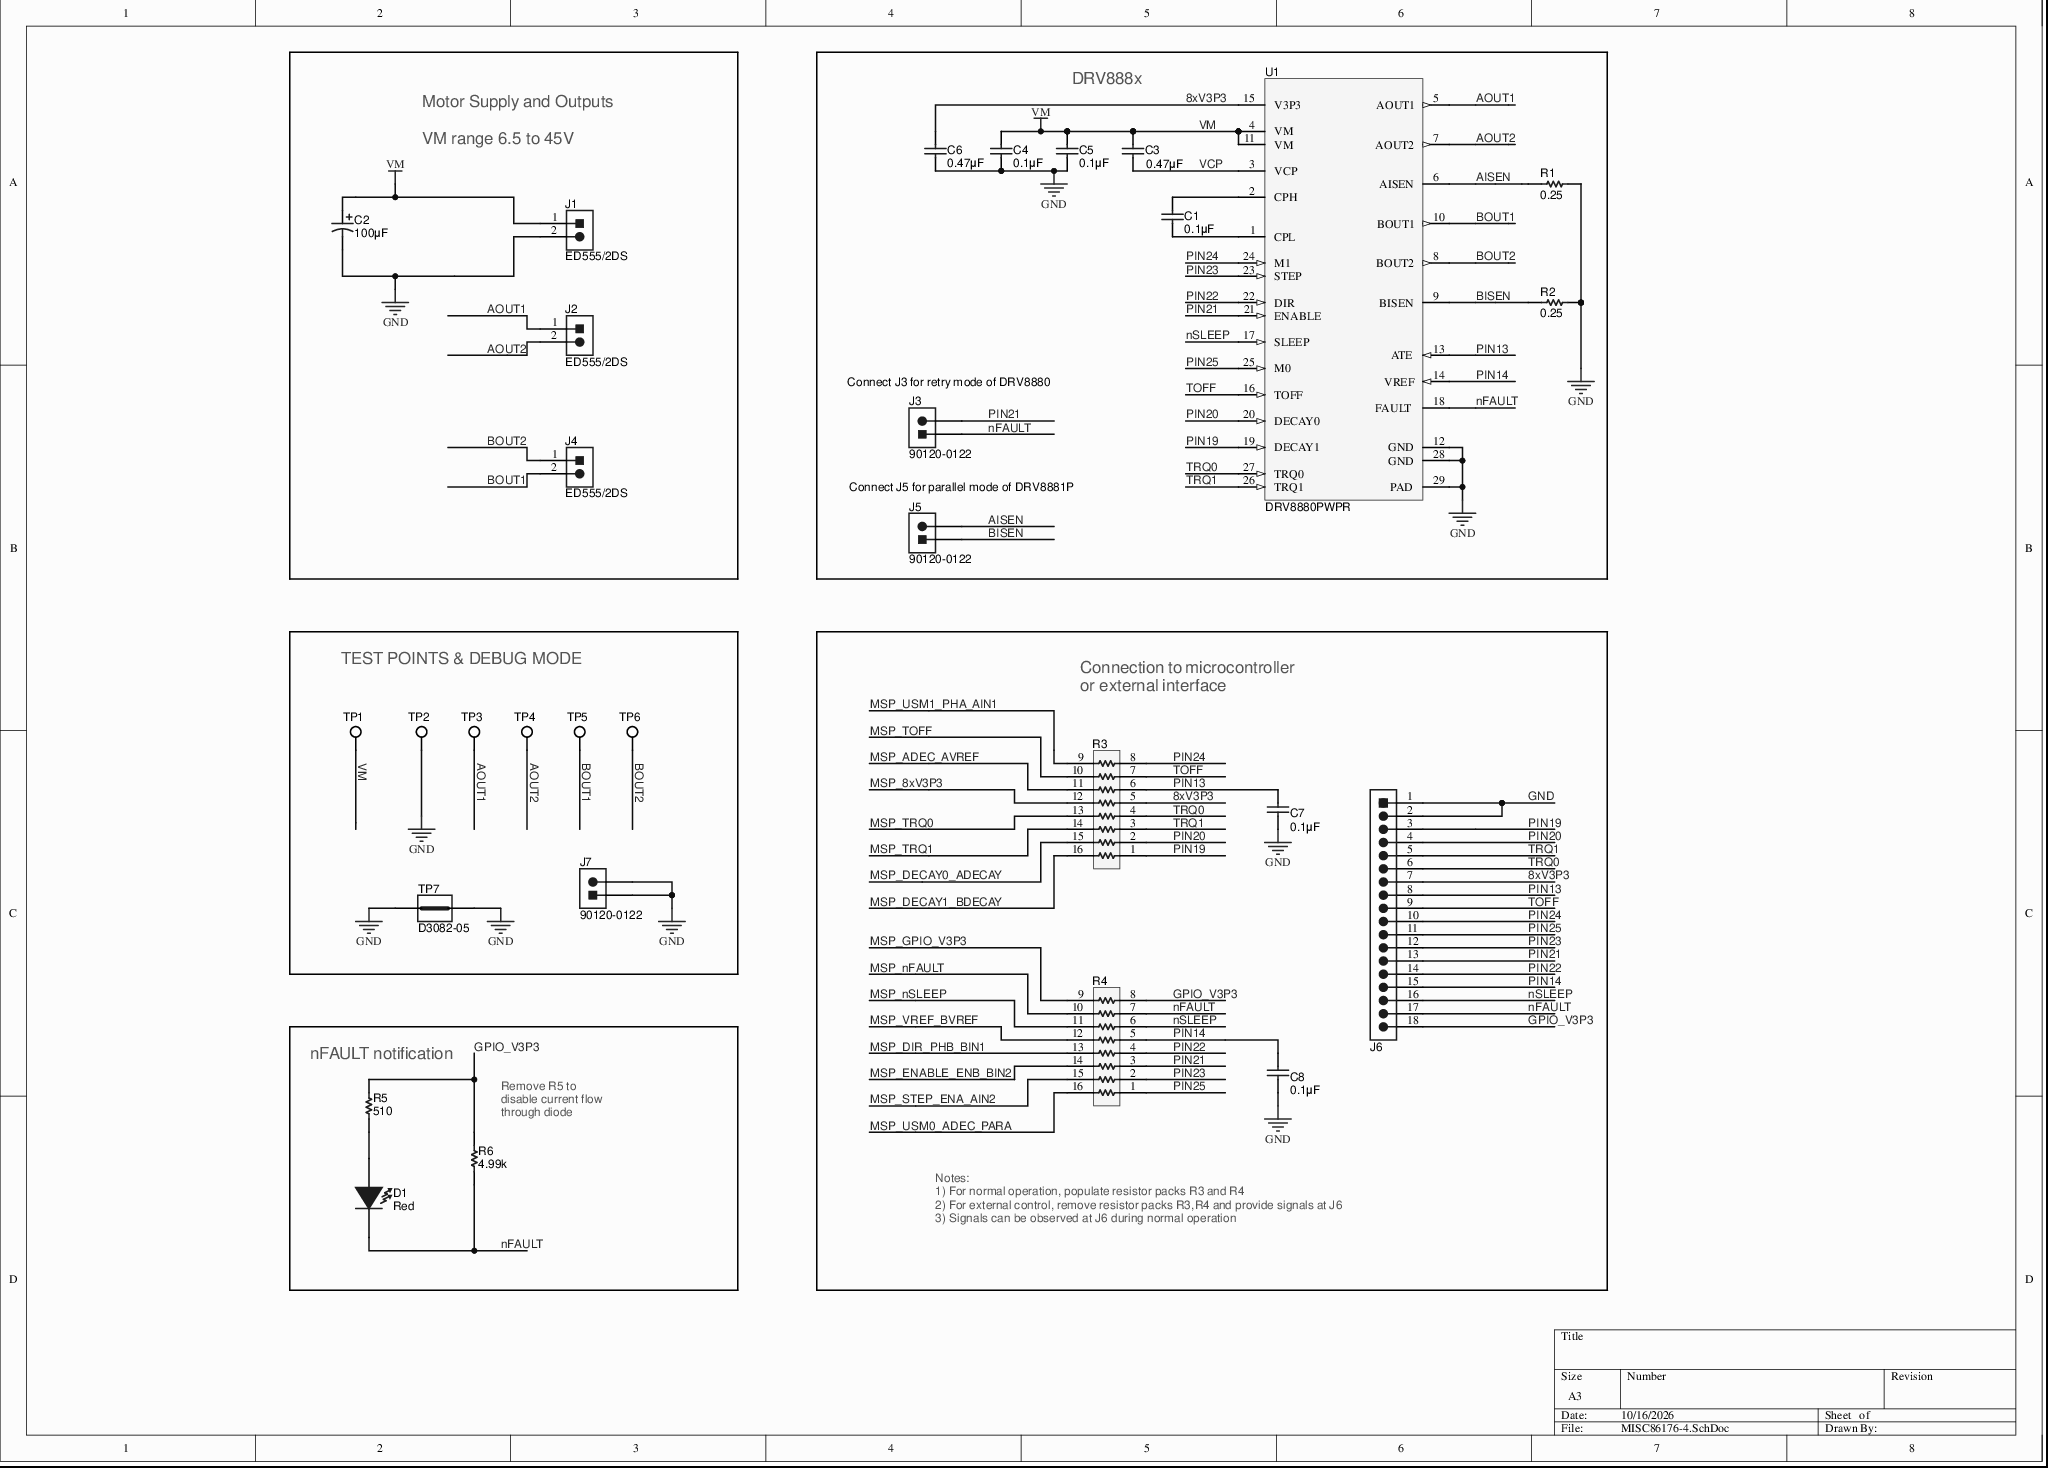
[diagram p0: MISC86176-4.SchDoc]
# Altium project MISC86176-2.PrjPCB
2 sheets, 47 parts. Net scope: global (net labels, ports and power ports of the same name join across sheets).
Board file: MISC86176.PcbDoc
Sheets:
  MISC86176-4.SchDoc
  MISC86176-6.SchDoc

## Sheet MISC86176-4.SchDoc
size A3

### Parts
C1  ValueDisplayed: 0.1µF  [0805L]  (hidden comment: C0805C104K1RACTU)
C2  ValueDisplayed: 100µF  [SM_RADIAL_G]  (hidden comment: EEE-FK1J101P)
C3  ValueDisplayed: 0.47µF  [0805L]  (hidden comment: C2012X7R1E474K)
C4  ValueDisplayed: 0.1µF  [0805L]  (hidden comment: C0805C104K1RACTU)
C5  ValueDisplayed: 0.1µF  [0805L]  (hidden comment: C0805C104K1RACTU)
C6  ValueDisplayed: 0.47µF  [0603L]  (hidden comment: C0603C474K9RACTU)
C7  ValueDisplayed: 0.1µF  [0402L]  (hidden comment: GRM155R61A104KA01D)
C8  ValueDisplayed: 0.1µF  [0402L]  (hidden comment: GRM155R61A104KA01D)
D1  value Red  [LED_LTST-C190_Red]  (hidden comment: LTST-C190CKT)
J1  ED555/2DS  [TERM_BLK_ED555-2DS]
J2  ED555/2DS  [TERM_BLK_ED555-2DS]
J3  90120-0122  [CONN_90120-0122]
J4  ED555/2DS  [TERM_BLK_ED555-2DS]
J5  90120-0122  [CONN_90120-0122]
J6  TSW-118-07-G-S  [TSW-118-07-G-S]  (value not drawn)
J7  90120-0122  [CONN_90120-0122]
R1  value 0.25  [2010L]  (hidden comment: CSRN2010FKR250)
R2  value 0.25  [2010L]  (hidden comment: CSRN2010FKR250)
R3  EXB-2HV330JV  [RESCAXS_EXB-2HV]  (value not drawn)
R4  EXB-2HV330JV  [RESCAXS_EXB-2HV]  (value not drawn)
R5  value 510  [0402L]  (hidden comment: CRCW0402510RJNED)
R6  value 4.99k  [0402L]  (hidden comment: CRCW04024K99FKED)
TP1  5016  [Testpoint_Keystone_Compact]  (value not drawn)
TP2  5016  [Testpoint_Keystone_Compact]  (value not drawn)
TP3  5016  [Testpoint_Keystone_Compact]  (value not drawn)
TP4  5016  [Testpoint_Keystone_Compact]  (value not drawn)
TP5  5016  [Testpoint_Keystone_Compact]  (value not drawn)
TP6  5016  [Testpoint_Keystone_Compact]  (value not drawn)
TP7  D3082-05  [Harwin_D3082-05]
U1  DRV8880PWPR  [PWP0028C_N]

### Blocks framed on the sheet
DRV888x: C1 C3-C6 J3 J5 R1 R2 U1
TEST POINTS & DEBUG MODE: J7 TP1-TP7
nFAULT notification: D1 R5 R6

### Nets
GND: C2.2(-) C4.1 C5.1 C6.2 C7.2 C8.2 J1.2 J6.1 J6.2 J7.1 J7.2 R1.1 R2.1 TP2.1 TP7.1 TP7.2 U1.12(GND) U1.28(GND) U1.29(PAD)
VM: C2.1(+) C3.2 C4.2 C5.2 J1.1 TP1.1 U1.4(VM) U1.11(VM)
8xV3P3: C6.1 J6.7 R3.5 U1.15(V3P3)
AISEN: J5.2 R1.2 U1.6(AISEN)
AOUT1: J2.1 TP3.1 U1.5(AOUT1)
AOUT2: J2.2 TP4.1 U1.7(AOUT2)
BISEN: J5.1 R2.2 U1.9(BISEN)
BOUT1: J4.2 TP5.1 U1.10(BOUT1)
BOUT2: J4.1 TP6.1 U1.8(BOUT2)
GPIO_V3P3: J6.18 R4.8 R5.2 R6.2
MSP_8xV3P3: R3.12
MSP_ADEC_AVREF: R3.11
MSP_DECAY0_ADECAY: R3.15
MSP_DECAY1_BDECAY: R3.16
MSP_DIR_PHB_BIN1: R4.13
MSP_ENABLE_ENB_BIN2: R4.14
MSP_GPIO_V3P3: R4.9
MSP_nFAULT: R4.10
MSP_nSLEEP: R4.11
MSP_STEP_ENA_AIN2: R4.15
MSP_TOFF: R3.10
MSP_TRQ0: R3.13
MSP_TRQ1: R3.14
MSP_USM0_ADEC_PARA: R4.16
MSP_USM1_PHA_AIN1: R3.9
MSP_VREF_BVREF: R4.12
nFAULT: D1.2(K) J3.1 J6.17 R4.7 R6.1 U1.18(~{FAULT})
nSLEEP: J6.16 R4.6 U1.17(~{SLEEP})
PIN13: C7.1 J6.8 R3.6 U1.13(ATE)
PIN14: C8.1 J6.15 R4.5 U1.14(VREF)
PIN19: J6.3 R3.1 U1.19(DECAY1)
PIN20: J6.4 R3.2 U1.20(DECAY0)
PIN21: J3.2 J6.13 R4.3 U1.21(ENABLE)
PIN22: J6.14 R4.4 U1.22(DIR)
PIN23: J6.12 R4.2 U1.23(STEP)
PIN24: J6.10 R3.8 U1.24(M1)
PIN25: J6.11 R4.1 U1.25(M0)
TOFF: J6.9 R3.7 U1.16(TOFF)
TRQ0: J6.6 R3.4 U1.27(TRQ0)
TRQ1: J6.5 R3.3 U1.26(TRQ1)
VCP: C3.1 U1.3(VCP)
NetC1_1: C1.1 U1.1(CPL)
NetC1_2: C1.2 U1.2(CPH)
NetD1_1: D1.1(A) R5.1

### Notes on the sheet
- Motor Supply and Outputs
  VM range 6.5 to 45V
- (near J3) Connect J3 for retry mode of DRV8880
- Connect J5 for parallel mode of DRV8881P
- Connection to microcontroller
  or external interface
- (near R6) Remove R5 to disable current flow through diode
- Notes:
  1) For normal operation, populate resistor packs R3 and R4
  2) For external control, remove resistor packs R3,R4 and provide signals at J6
  3) Signals can be observed at J6 during normal operation

### Library data of the parts
C1 C4 C5 = C0805C104K1RACTU: CAP, CERM, 0.1 µF, 100 V, +/- 10%, X7R, 0805; Manufacturer: Kemet; Polarized: N; CompType: Capacitor; Value: 0.1uF; U/M: EA; Cap_F: 0.0000001; Tolerance_%: 10; ESR_ohm: 0.064; Value1: 0.064 ohm; VDC_V: 100; Value2: 100V; IRMS_A: 1.64; TaMin_C: -55; TaMax_C: 125; Cap_Case: 0805; SymbolVersion: 2008-07-09; PartNumber: C0805C104K1RACTU; PackageReference: 0805; RoHS: Y; MountType: SMT; Technology: Ceramic; TempCo: X7R; Published: 2008-06-19; LatestRevisionDate: 2015-06-10; ComponentLink1Description: Datasheet link; ComponentLink1URL: http://www.kemet.com/kemet/web/homepage/kechome.nsf/file/Partial%20Copy%20-%20Ceramic%20Surface%20Mount%20Capacitors/$file/F3102_CE.pdf; Supplier 1: Digi-Key; Supplier Part Number 1: 399-3486-1-ND; Supplier 2: Mouser; Supplier Part Number 2: 80-C0805C104K1R; Supplier 3: Farnell; Supplier Part Number 3: 1650862; Publisher: Texas Instruments
C2 = EEE-FK1J101P: CAP, AL, 100 µF, 63 V, +/- 20%, 0.35 ohm, SMD; Manufacturer: Panasonic; Value: 100uF; Polarized: Y; CompType: Capacitor; U/M: EA; Cap_F: 0.0001; Tolerance_%: 20; ESR_ohm: 0.35; VDC_V: 63; Value2: 63V; IRMS_A: 0.4; TaMin_C: -55; TaMax_C: 105; Cap_Case: G; SymbolVersion: 2008-07-09; PartNumber: EEE-FK1J101P; PackageReference: SMT Radial G; RoHS: Y; Value1: 0.35 ohm; MountType: SMT; Technology: AL; LatestRevisionDate: 2015-06-10; ComponentLink1Description: Datasheet link; ComponentLink1URL: http://www.panasonic.com/industrial/components/pdf/smt_aec_050505.pdf; Supplier 1: Digi-Key; Supplier Part Number 1: PCE3819CT-ND; Supplier 2: Mouser; Supplier Part Number 2: 667-EEE-FK1J101P; Supplier 3: Farnell; Supplier Part Number 3: 9696040; Series: FK; Publisher: Texas Instruments
C3 = C2012X7R1E474K: CAP, CERM, 0.47 µF, 25 V, +/- 10%, X7R, 0805; Manufacturer: TDK; Polarized: N; CompType: Capacitor; Value: 0.47uF; U/M: EA; Cap_F: 0.00000047; Tolerance_%: 10; ESR_ohm: 0.0101; Value1: 0.0101 ohm; VDC_V: 25; Value2: 25V; TaMin_C: -55; TaMax_C: 125; Cap_Case: 0805; SymbolVersion: 2008-07-09; PartNumber: C2012X7R1E474K; PackageReference: 0805; RoHS: Y; MountType: SMT; Technology: Ceramic; TempCo: X7R; Published: 2008-06-19; LatestRevisionDate: 2015-06-10; ComponentLink1Description: Datasheet link; ComponentLink1URL: http://www.tdk.co.jp/tefe02/e412_c.pdf; Supplier 1: Digi-Key; Supplier Part Number 1: 445-1353-1-ND; Supplier 2: Farnell; Supplier Part Number 2: 1844282; Publisher: Texas Instruments
C6 = C0603C474K9RACTU: CAP, CERM, 0.47 µF, 6.3 V, +/- 10%, X7R, 0603; Manufacturer: Kemet; Polarized: N; CompType: Capacitor; Value: 0.47uF; U/M: EA; Cap_F: 0.00000047; Tolerance_%: 10; Value1: Unknown; VDC_V: 6.3; Value2: 6.3V; TaMin_C: -55; TaMax_C: 125; Cap_Case: 0603; SymbolVersion: 2008-07-09; PartNumber: C0603C474K9RACTU; PackageReference: 0603; RoHS: Y; MountType: SMT; Technology: Ceramic; TempCo: X7R; Published: 2008-06-19; LatestRevisionDate: 2015-06-10; ComponentLink1Description: Datasheet link; ComponentLink1URL: http://www.kemet.com/kemet/web/homepage/kechome.nsf/vapubfiles/F3102_Y5V.pdf/$file/F3102_Y5V.pdf; Supplier 1: Digi-Key; Supplier Part Number 1: 399-4924-1-ND; Supplier 2: Mouser; Supplier Part Number 2: 80-C0603C474K9R; Publisher: Texas Instruments
C7 C8 = GRM155R61A104KA01D: CAP, CERM, 0.1 µF, 10 V, +/- 10%, X5R, 0402; Manufacturer: MuRata; Value: 0.1uF; Polarized: N; CompType: Capacitor; U/M: EA; Cap_F: 0.0000001; Tolerance_%: 10; Value1: Unknown; Value2: 10V; TaMin_C: -55; TaMax_C: 85; Cap_Case: 0402; SymbolVersion: 2008-07-09; PartNumber: GRM155R61A104KA01D; PackageReference: 0402; RoHS: Y; VDC_V: 10; MountType: SMT; Technology: Ceramic; TempCo: X5R; Published: 2008-06-19; LatestRevisionDate: 2015-06-10; ComponentLink1Description: Datasheet link; ComponentLink1URL: http://search.murata.co.jp/Ceramy/PnsearchViewAction.do?HnOFG=ON&HnNFG=ON&SEL_CNT=50&sLang=en&sKey=GRM155R61A104KA01D&x=9&y=9&search=startwith; Supplier 1: Digi-Key; Supplier Part Number 1: 490-1318-1-ND; Supplier 2: Mouser; Supplier Part Number 2: 81-GRM155R61A104KA01; Supplier 3: Farnell; Supplier Part Number 3: 1828862; Publisher: Texas Instruments
D1 = LTST-C190CKT: LED, Red, SMD; Manufacturer: Lite-On; Vf_V: 2; Value2: 2V; Io_A: 0.02; Tjmax_C: 85; Power_TotalModule: 0.0625; Value1: 0.0625W; U/M: EA; ComponentLink1URL: http://optoelectronics.liteon.com/en-us/api/DwonloadFileHandler.ashx?txtSpecNo=DS-22-98-0009&txtPartNo=LTST-C190CKT; SymbolVersion: 2008-12-08; PackageReference: Red LED, 1.6x0.8x0.8mm; PartNumber: LTST-C190CKT; ComponentLink1Description: Datasheet link; Supplier 1: Digi-Key; Supplier Part Number 1: 160-1181-1-ND; MountType: SMT; CompType: LED; RoHS: Y; Type: ?; Color: red; Published: 2008-07-11; LatestRevisionDate: 2015-06-04; Supplier 2: Mouser; Supplier Part Number 2: 859-LTST-C190CKT; Publisher: Texas Instruments
J1 J2 J4 = ED555/2DS: Terminal Block, 6A, 3.5mm Pitch, 2-Pos, TH; Manufacturer: On-Shore Technology; CompType: Connector; U/M: EA; ComponentLink1URL: http://on-shore.com/sites/default/files/manuals/ed555ds.pdf; SymbolVersion: 2013-10-31; PackageReference: 7.0x8.2x6.5mm; PartNumber: ED555/2DS; ComponentLink1Description: Datasheet Link; RoHS: Y; MountType: TH; LatestRevisionDate: 2015-06-10; Supplier 1: Digi-Key; Supplier Part Number 1: ED1514-ND; Publisher: Texas Instruments
J3 J5 J7 = 90120-0122: Header, 100mil, 2x1, Tin, TH; Manufacturer: Molex; U/M: EA; SymbolVersion: 2013-10-31; PartNumber: 90120-0122; PackageReference: Header 2x1; CompType: Header; RoHS: Y; MountType: TH; ComponentLink1Description: Datasheet Link; ComponentLink1URL: http://www.molex.com/pdm_docs/sd/901200122_sd.pdf; LatestRevisionDate: 2015-06-11; Supplier 1: Digi-Key; Supplier Part Number 1: WM8072-ND; Supplier 2: Mouser; Supplier Part Number 2: 538-90120-0122; Supplier 3: Newark; Supplier Part Number 3: 19M8215; ClassName: Header; Publisher: Texas Instruments
J6 = TSW-118-07-G-S: Header, 100mil, 18x1, Gold, TH; Manufacturer: Samtec; U/M: EA; SymbolVersion: 2013-12-22; PackageReference: 18x1 Header; PartNumber: TSW-118-07-G-S; ComponentLink1Description: Datasheet Link; Supplier 1: Digi-Key; Supplier Part Number 1: SAM1029-18-ND; MountType: TH; ClassName: Header; CompType: Header; RoHS: Y; LatestRevisionDate: 2015-06-08; Publisher: Texas Instruments
R1 R2 = CSRN2010FKR250: RES, 0.25, 1%, 1 W, 2010; Manufacturer: Stackpole Electronics Inc; CompType: Resistor; Value_Code: R250; Tolerance_%: 1; Value2: 1W; TempCo: 250 ppm/C; U/M: EA; SymbolVersion: 2009-05-29; PartNumber: CSRN2010FKR250; PackageReference: 2010; RoHS: Y; Res_ohm: 0.25; Value1: 1%; Power_W: 1; MountType: SMT; Technology: Thick Film; Published: 2008-06-26; LatestRevisionDate: 2015-04-13; ComponentLink1Description: Datasheet link; Supplier 1: Digi-Key; Supplier Part Number 1: CSRN2010FKR250CT-ND; ValueDisplayed: 0.25; Publisher: Texas Instruments
R3 R4 = EXB-2HV330JV: RES, 33, 5%, 0.0625 W, Resistor Array - 8x1; Manufacturer: Panasonic; Res_ohm: 33; Value: 33; Value_Code: 33R0; Tolerance_%: 5; Power_W: 0.0625; TempCo: 200 ppm/C; EIA_Code: E24; U/M: EA; SymbolVersion: 2013-05-25; PartNumber: EXB-2HV330JV; PackageReference: Resistor Array - 8x1; RoHS: Y; CompType: Resistor; Value1: 5%; Value2: 0.0625W; MountType: SMT; Technology: Thick Film; Published: 2008-06-26; LatestRevisionDate: 2015-06-01; ComponentLink1Description: Datasheet link; ComponentLink1URL: http://industrial.panasonic.com/www-data/pdf/AOC0000/AOC0000CE1.pdf; Supplier 1: Digi-Key; Supplier Part Number 1: Y1330CT-ND; Supplier 2: Mouser; Supplier Part Number 2: 667-EXB-2HV330JV; Supplier 3: Farnell; Supplier Part Number 3: 2060066; ValueDisplayed: 33; Publisher: Texas Instruments
R5 = CRCW0402510RJNED: RES, 510, 5%, 0.063 W, 0402; Manufacturer: Vishay-Dale; CompType: Resistor; Value_Code: 510R; Tolerance_%: 5; Power_W: 0.063; Value2: 0.063W; VDC_V: 50; TempCo: 200 ppm/C; EIA_Code: E24; U/M: EA; SymbolVersion: 2009-05-29; PartNumber: CRCW0402510RJNED; PackageReference: 0402; RoHS: Y; Res_ohm: 510; Value1: 5%; MountType: SMT; Technology: Thick Film; Published: 2008-06-26; LatestRevisionDate: 2015-05-27; ComponentLink1Description: Datasheet link; ComponentLink1URL: http://www.vishay.com/docs/20035/dcrcwe3.pdf; Supplier 1: Digi-Key; Supplier Part Number 1: 541-510JCT-ND; Supplier 2: Mouser; Supplier Part Number 2: 71-CRCW0402J-510-E3; Supplier 3: Farnell; Supplier Part Number 3: 1570682; ValueDisplayed: 510; Publisher: Texas Instruments
R6 = CRCW04024K99FKED: RES, 4.99 k, 1%, 0.063 W, 0402; Manufacturer: Vishay-Dale; CompType: Resistor; Res_ohm: 4990; Value_Code: 4k99; Tolerance_%: 1; Power_W: 0.063; Value2: 0.063W; VDC_V: 50; TempCo: 100 ppm/C; EIA_Code: E96; U/M: EA; SymbolVersion: 2009-05-29; PartNumber: CRCW04024K99FKED; PackageReference: 0402; RoHS: Y; Value1: 1%; MountType: SMT; Technology: Thick Film; Published: 2008-06-26; LatestRevisionDate: 2015-05-27; ComponentLink1Description: Datasheet link; ComponentLink1URL: http://www.vishay.com/docs/20035/dcrcwe3.pdf; Supplier 1: Digi-Key; Supplier Part Number 1: 541-4.99KLCT-ND; Supplier 2: Mouser; Supplier Part Number 2: 71-CRCW0402-4.99K-E3; Supplier 3: Farnell; Supplier Part Number 3: 1469715; ValueDisplayed: 4.99k; Publisher: Texas Instruments
TP1-TP6 = 5016: Test Point, Compact, SMT; Manufacturer: Keystone; CompType: Test Point Loop; U/M: EA; SymbolVersion: 2008-04-04; PartNumber: 5016; Value: SMT; RoHS: Y; PackageReference: Testpoint_Keystone_Compact; MountType: SMT; ComponentLink1Description: Datasheet Link; ComponentLink1URL: http://www.keyelco.com/userAssets/store/files/5016.PDF; LatestRevisionDate: 2015-05-13; Supplier 1: Digi-Key; Supplier Part Number 1: 5016KCT-ND; Publisher: Texas Instruments
TP7 = D3082-05: 1mm Uninsulated Shorting Plug, 10.16mm spacing, TH; Manufacturer: Harwin; CompType: Jumper Wire; U/M: EA; SymbolVersion: 2014-05-16; MountType: TH; RoHS: Y; PartNumber: D3082-05; PackageReference: Shorting Plug, 10.16mm spacing, TH; ComponentLink1Description: Datasheet Link; ComponentLink1URL: http://cdn.harwin.com/pdfs/D3080-D3083.pdf; Supplier 1: Digi-Key; Supplier 2: Mouser; Supplier Part Number 1: 952-1873-ND; Supplier Part Number 2: 855-D3082-05; LatestRevisionDate: 2015-06-10; Publisher: Texas Instruments
U1 = DRV8880PWPR: 2-A 45-V 1/16-µstep Stepper Motor Driver With AutoTune, PWP0028C; Manufacturer: Texas Instruments; SymbolCreator: Altium; CompType: IC; U/M: EA; SymbolVersion: 2015-05-04; PartNumber: DRV8880PWPR; Alternate PartNumber: DRV8880PWP; PackageReference: PWP0028C; MountType: SMT; ComponentLink1Description: Datasheet Link; LatestRevisionDate: 2015-06-11; Alternate Manufacturer: Texas Instruments; Publisher: Texas Instruments

## Sheet MISC86176-6.SchDoc
size A2
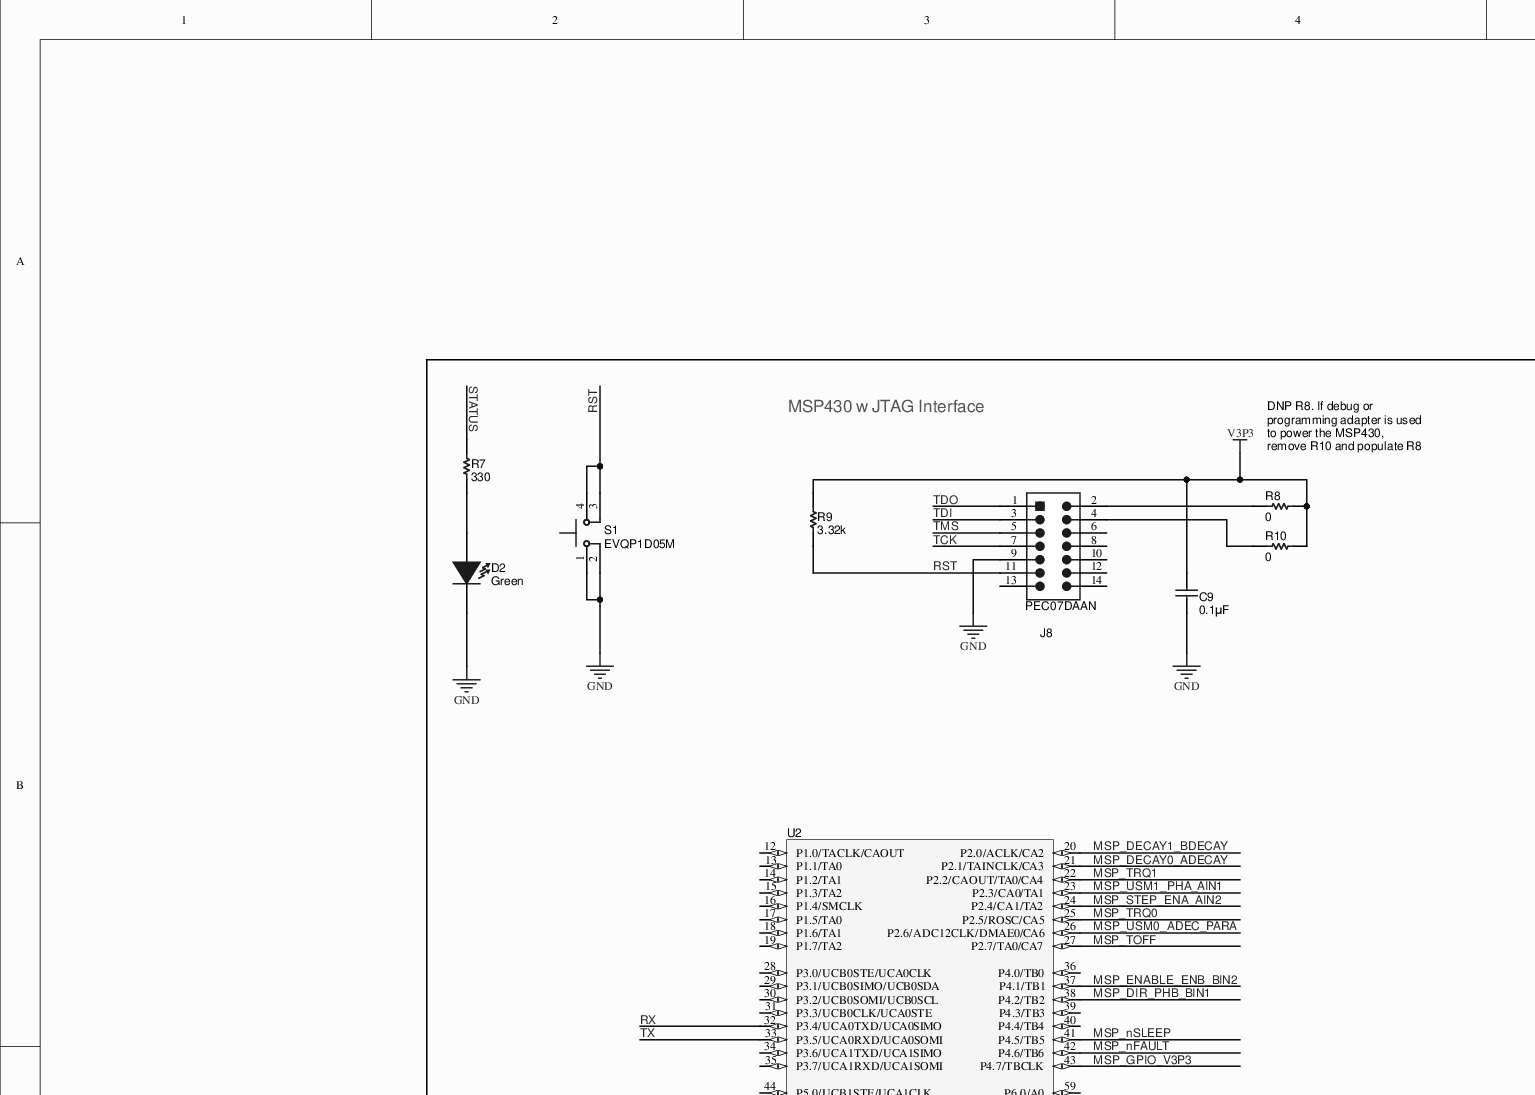
[diagram p1: MISC86176-6.SchDoc, top left]
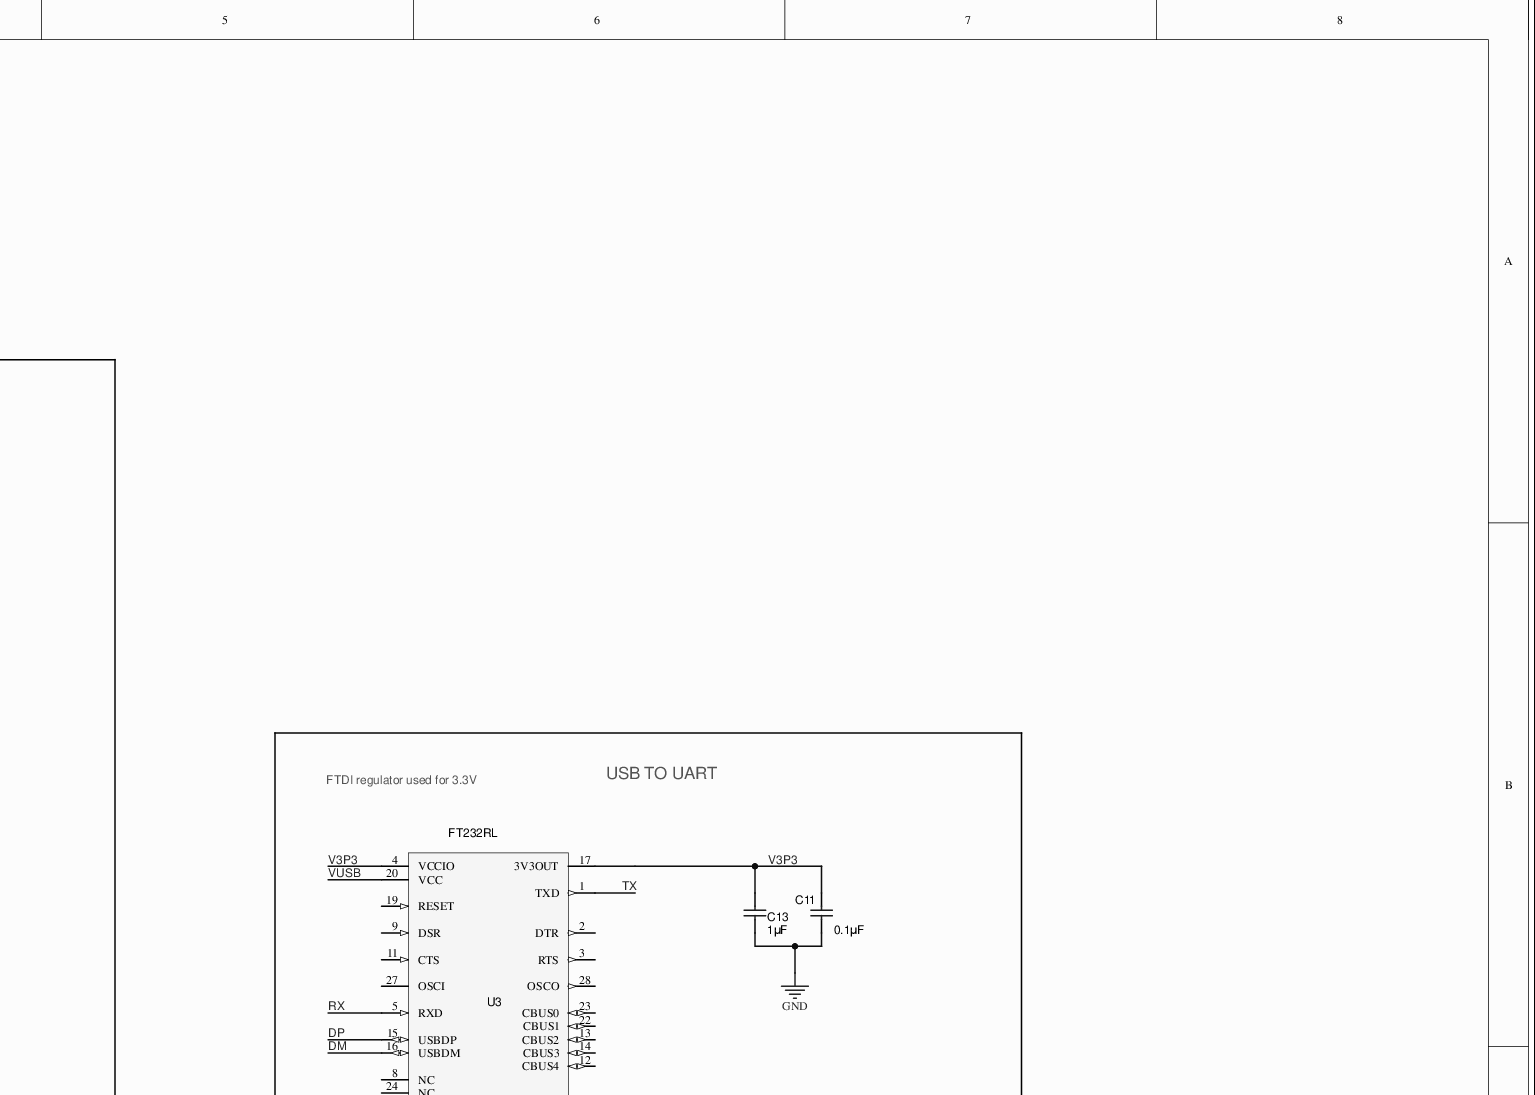
[diagram p2: MISC86176-6.SchDoc, top right]
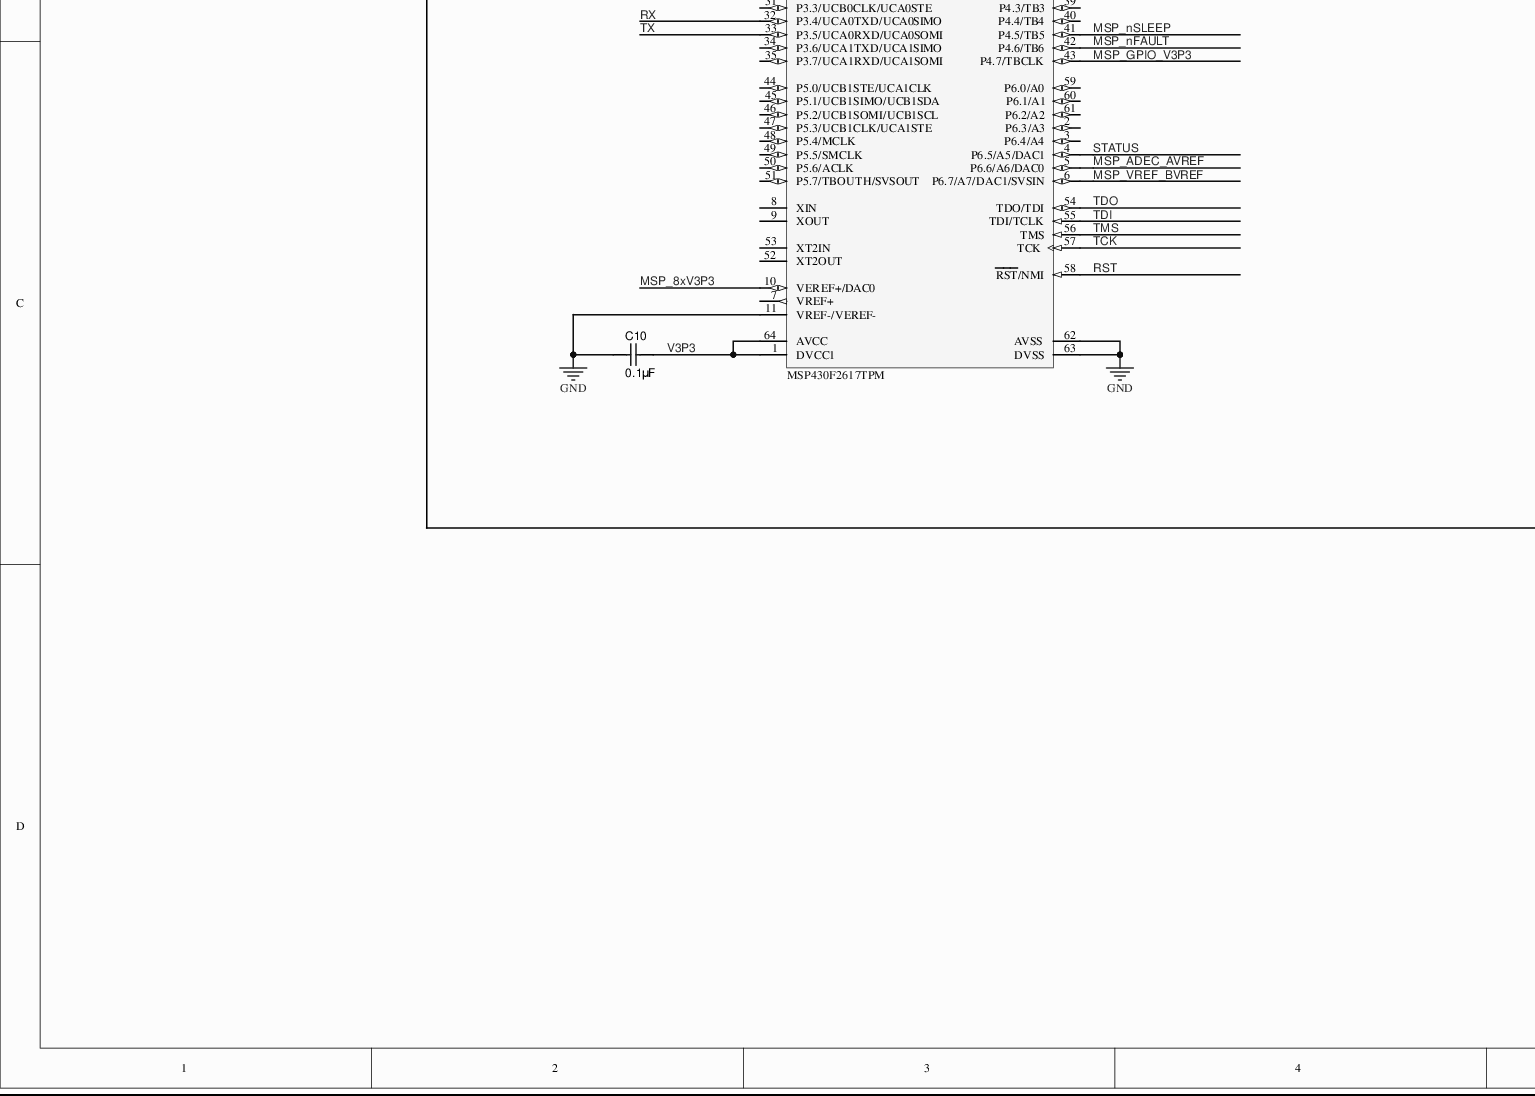
[diagram p3: MISC86176-6.SchDoc, bottom left]
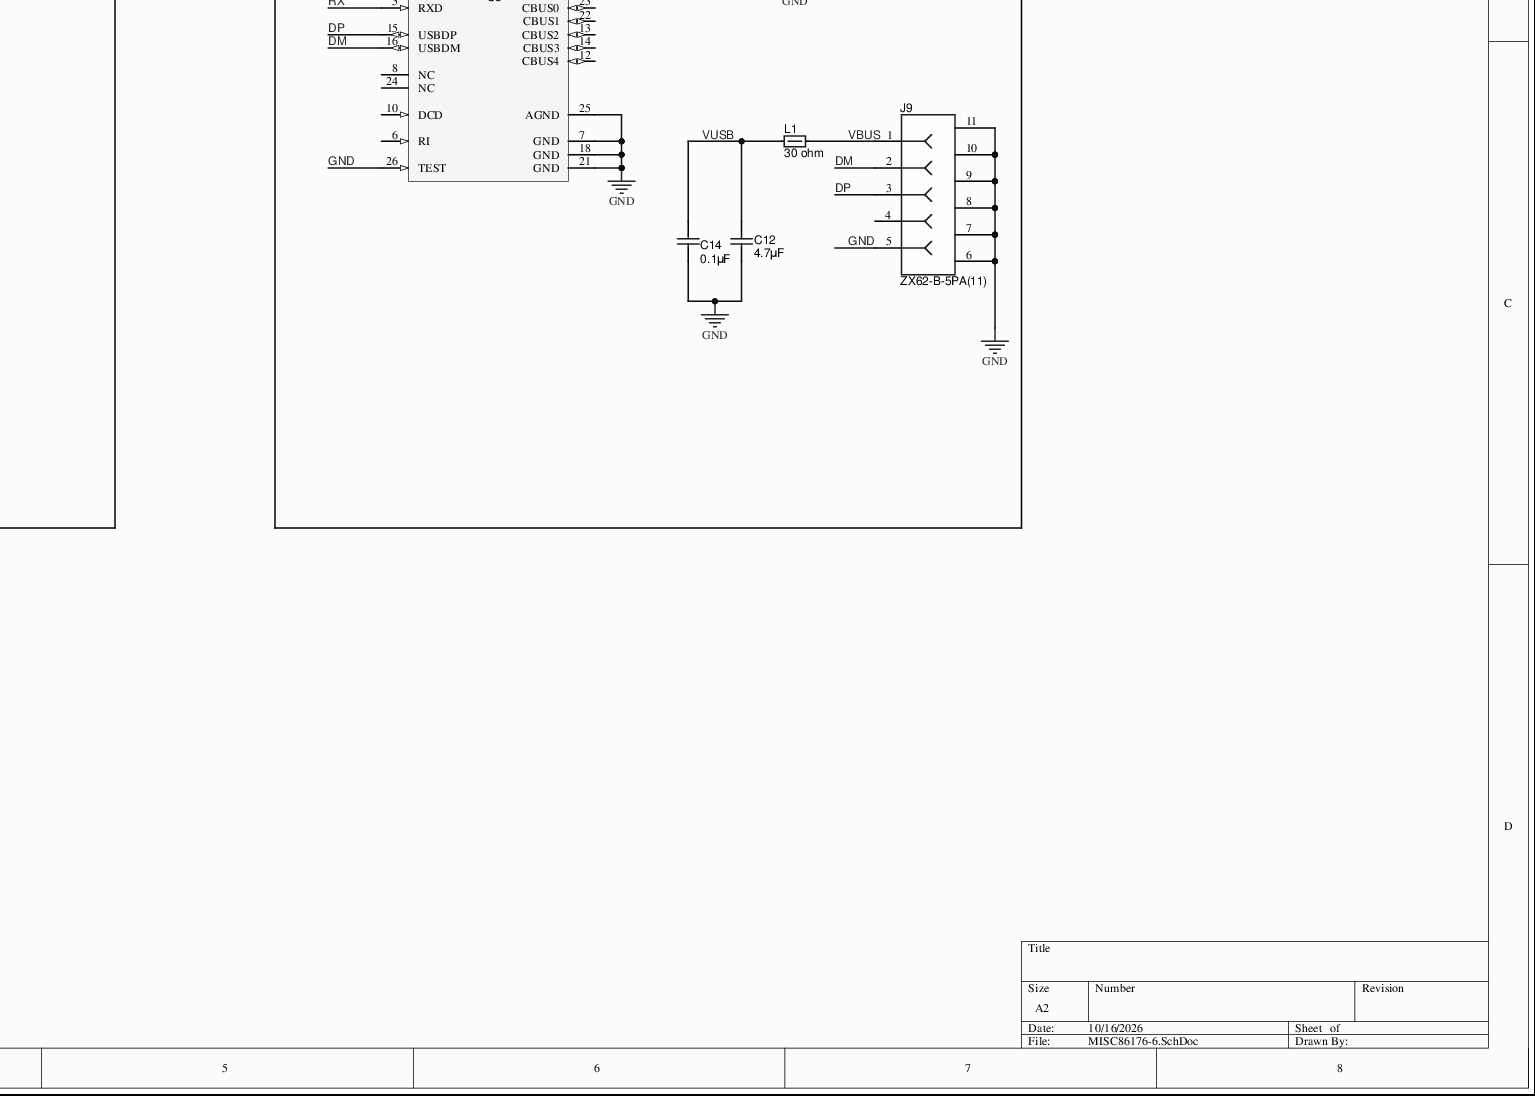
[diagram p4: MISC86176-6.SchDoc, bottom right]

### Parts
C9  ValueDisplayed: 0.1µF  [0402L]  (hidden comment: GRM155R61A104KA01D)
C10  ValueDisplayed: 0.1µF  [0402L]  (hidden comment: GRM155R61A104KA01D)
C11  ValueDisplayed: 0.1µF  [0402L]  (hidden comment: GRM155R61A104KA01D)
C12  ValueDisplayed: 4.7µF  [0603L]  (hidden comment: CGB3B1X5R1A475K055AC)
C13  ValueDisplayed: 1µF  [0402L]  (hidden comment: GRM155R61A105KE15D)
C14  ValueDisplayed: 0.1µF  [0402L]  (hidden comment: GRM155R61A104KA01D)
D2  value Green  [LED_LTST-C190]  (hidden comment: LTST-C190GKT)
J8  PEC07DAAN  [CONN_PEC07DAAN]
J9  ZX62-B-5PA(11)  [CONN_USB_micro_ZX62-B-5PA]
L1  value 30 ohm  [0805L]  (hidden comment: MMZ2012R300A)
R7  value 330  [0402L]  (hidden comment: CRCW0402330RJNED)
R8  value 0  [0402L]  (hidden comment: ERJ-2GE0R00X)
R9  value 3.32k  [0402L]  (hidden comment: CRCW04023K32FKED)
R10  value 0  [0402L]  (hidden comment: ERJ-2GE0R00X)
S1  EVQP1D05M  [SW_EVQxxx05M]
U2  MSP430F2617TPM  [PM0064A_L]
U3  FT232RL  [SSOP28_M]

### Blocks framed on the sheet
MSP430 w JTAG Interface: C9 C10 D2 J8 R7-R10 S1 U2
USB TO UART: C11-C14 J9 L1 U3

### Nets
GND: C9.2 C10.2 C11.2 C12.2 C13.2 C14.2 D2.2(K) J8.9 J9.5 J9.6 J9.7 J9.8 J9.9 J9.10 J9.11 S1.1 S1.2 U2.11(VREF-/VEREF-) U2.62(AVSS) U2.63(DVSS) U3.7(GND) U3.18(GND) U3.21(GND) U3.25(AGND) U3.26(TEST)
V3P3: C9.1 C10.1 C11.1 C13.1 R8.1 R9.2 R10.1 U2.1(DVCC1) U2.64(AVCC) U3.4(VCCIO) U3.17(3V3OUT)
DM: J9.2 U3.16(USBDM)
DP: J9.3 U3.15(USBDP)
MSP_8xV3P3: U2.10(VEREF+/DAC0)
MSP_ADEC_AVREF: U2.5(P6.6/A6/DAC0)
MSP_DECAY0_ADECAY: U2.21(P2.1/TAINCLK/CA3)
MSP_DECAY1_BDECAY: U2.20(P2.0/ACLK/CA2)
MSP_DIR_PHB_BIN1: U2.38(P4.2/TB2)
MSP_ENABLE_ENB_BIN2: U2.37(P4.1/TB1)
MSP_GPIO_V3P3: U2.43(P4.7/TBCLK)
MSP_nFAULT: U2.42(P4.6/TB6)
MSP_nSLEEP: U2.41(P4.5/TB5)
MSP_STEP_ENA_AIN2: U2.24(P2.4/CA1/TA2)
MSP_TOFF: U2.27(P2.7/TA0/CA7)
MSP_TRQ0: U2.25(P2.5/ROSC/CA5)
MSP_TRQ1: U2.22(P2.2/CAOUT/TA0/CA4)
MSP_USM0_ADEC_PARA: U2.26(P2.6/ADC12CLK/DMAE0/CA6)
MSP_USM1_PHA_AIN1: U2.23(P2.3/CA0/TA1)
MSP_VREF_BVREF: U2.6(P6.7/A7/DAC1/SVSIN)
RST: J8.11 R9.1 S1.3 S1.4 U2.58(~{RST}/NMI)
RX: U2.32(P3.4/UCA0TXD/UCA0SIMO) U3.5(RXD)
STATUS: R7.2 U2.4(P6.5/A5/DAC1)
TCK: J8.7 U2.57(TCK)
TDI: J8.3 U2.55(TDI/TCLK)
TDO: J8.1 U2.54(TDO/TDI)
TMS: J8.5 U2.56(TMS)
TX: U2.33(P3.5/UCA0RXD/UCA0SOMI) U3.1(TXD)
VBUS: J9.1 L1.2
VUSB: C12.1 C14.1 L1.1 U3.20(VCC)
NetD2_1: D2.1(A) R7.1
NetJ8_2: J8.2 R8.2
NetJ8_4: J8.4 R10.2

Not connected (* = marked no-connect by the designer): J8 6* 8* 10* 12* 13* 14*; J9 4*; U2 2(P6.3/A3)* 3(P6.4/A4)* 7(VREF+)* 8(XIN)* 9(XOUT)* 12(P1.0/TACLK/CAOUT)* 13(P1.1/TA0)* 14(P1.2/TA1)* 15(P1.3/TA2)* 16(P1.4/SMCLK)* 17(P1.5/TA0)* 18(P1.6/TA1)* 19(P1.7/TA2)* 28(P3.0/UCB0STE/UCA0CLK)* 29(P3.1/UCB0SIMO/UCB0SDA)* 30(P3.2/UCB0SOMI/UCB0SCL)* 31(P3.3/UCB0CLK/UCA0STE)* 34(P3.6/UCA1TXD/UCA1SIMO)* 35(P3.7/UCA1RXD/UCA1SOMI)* 36(P4.0/TB0)* 39(P4.3/TB3)* 40(P4.4/TB4)* 44(P5.0/UCB1STE/UCA1CLK)* 45(P5.1/UCB1SIMO/UCB1SDA)* 46(P5.2/UCB1SOMI/UCB1SCL)* 47(P5.3/UCB1CLK/UCA1STE)* 48(P5.4/MCLK)* 49(P5.5/SMCLK)* 50(P5.6/ACLK)* 51(P5.7/TBOUTH/SVSOUT)* 52(XT2OUT)* 53(XT2IN)* 59(P6.0/A0)* 60(P6.1/A1)* 61(P6.2/A2)*; U3 2(~{DTR})* 3(~{RTS})* 6(~{RI})* 8(NC)* 9(~{DSR})* 10(~{DCD})* 11(~{CTS})* 12(CBUS4)* 13(CBUS2)* 14(CBUS3)* 19(~{RESET})* 22(CBUS1)* 23(CBUS0)* 24(NC)* 27(OSCI)* 28(OSCO)*

### Notes on the sheet
- (near R8) DNP R8. If debug or programming adapter is used to power the MSP430, remove R10 and populate R8
- FTDI regulator used for 3.3V

### Library data of the parts
C9-C11 C14 = GRM155R61A104KA01D: as C7 on sheet MISC86176-4; SymbolVersion: 2008-07-09; PartNumber: GRM155R61A104KA01D; PackageReference: 0402; RoHS: Y; VDC_V: 10; MountType: SMT; Technology: Ceramic; TempCo: X5R; Published: 2008-06-19; LatestRevisionDate: 2015-06-10; ComponentLink1Description: Datasheet link; ComponentLink1URL: http://search.murata.co.jp/Ceramy/PnsearchViewAction.do?HnOFG=ON&HnNFG=ON&SEL_CNT=50&sLang=en&sKey=GRM155R61A104KA01D&x=9&y=9&search=startwith; Supplier 1: Digi-Key; Supplier Part Number 1: 490-1318-1-ND; Supplier 2: Mouser; Supplier Part Number 2: 81-GRM155R61A104KA01; Supplier 3: Farnell; Supplier Part Number 3: 1828862; Publisher: Texas Instruments
C12 = CGB3B1X5R1A475K055AC: CAP, CERM, 4.7 µF, 10 V, +/- 10%, X5R, 0603; Manufacturer: TDK; Polarized: N; CompType: Capacitor; Value: 4.7uF; U/M: EA; Cap_F: 0.0000047; Tolerance_%: 10; Value1: Unknown; Value2: 10V; TaMin_C: -55; TaMax_C: 85; Cap_Case: 0603; SymbolVersion: 2008-07-09; PartNumber: CGB3B1X5R1A475K055AC; PackageReference: 0603; RoHS: Y; VDC_V: 10; MountType: SMT; Technology: Ceramic; TempCo: X5R; Published: 2008-06-19; LatestRevisionDate: 2015-06-10; ComponentLink1Description: Datasheet link; ComponentLink1URL: http://www.tdk.com/pdf/mlcc_product_guide_A12.pdf; Supplier 1: Digi-Key; Supplier Part Number 1: 445-7482-1-ND; Publisher: Texas Instruments
C13 = GRM155R61A105KE15D: CAP, CERM, 1 µF, 10 V, +/- 10%, X5R, 0402; Manufacturer: MuRata; Value: 1uF; Polarized: N; CompType: Capacitor; U/M: EA; Cap_F: 0.000001; Tolerance_%: 10; Value1: Unknown; Value2: 10V; TaMin_C: -55; TaMax_C: 85; Cap_Case: 0402; SymbolVersion: 2008-07-09; PartNumber: GRM155R61A105KE15D; PackageReference: 0402; RoHS: Y; VDC_V: 10; MountType: SMT; Technology: Ceramic; TempCo: X5R; Published: 2008-06-19; LatestRevisionDate: 2015-06-10; ComponentLink1Description: Datasheet link; ComponentLink1URL: http://search.murata.co.jp/Ceramy/PnsearchViewAction.do?HnOFG=ON&HnNFG=ON&SEL_CNT=50&sLang=en&sKey=GRM155R61A105KE15D&x=9&y=9&search=startwith; Supplier 1: Digi-Key; Supplier Part Number 1: 490-3890-1-ND; Supplier 2: Mouser; Supplier Part Number 2: 81-GRM155R61A105KE15; Supplier 3: Farnell; Supplier Part Number 3: 1735523; Publisher: Texas Instruments
D2 = LTST-C190GKT: LED, Green, SMD; Manufacturer: Lite-On; Vf_V: 2.1; Value2: 2.1V; Io_A: 0.02; Power_TotalModule: 0.1; Value1: 0.1W; U/M: EA; PartNumber: LTST-C190GKT; SymbolVersion: 2008-12-08; PackageReference: 1.6x0.8x0.8mm; ComponentLink1Description: Datasheet link; Supplier 1: Digi-Key; Supplier Part Number 1: 160-1183-1-ND; MountType: SMT; CompType: LED; RoHS: Y; Type: ?; Color: green; Published: 2008-07-11; LatestRevisionDate: 2015-06-04; Supplier 2: Mouser; Supplier Part Number 2: 859-LTST-C190GKT; Publisher: Texas Instruments
J8 = PEC07DAAN: Header, 100mil, 7x2, Tin, TH; Manufacturer: Sullins Connector Solutions; U/M: EA; SymbolVersion: 2013-12-22; PartNumber: PEC07DAAN; PackageReference: Header, 7x2, 100mil, Tin; CompType: Header; RoHS: Y; MountType: TH; ComponentLink1Description: Datasheet Link; ComponentLink1URL: http://www.sullinscorp.com/catalogs/97_Page78-79_HEADER_.100_2.54mm_MALE_BREAKAWAY.pdf; LatestRevisionDate: 2015-06-02; Supplier 1: Digi-Key; Supplier Part Number 1: S2012E-07-ND; ClassName: Header; Publisher: Texas Instruments
J9 = ZX62-B-5PA(11): Connector, Receptacle, Micro-USB Type B, R/A, Bottom Mount SMT; Manufacturer: Hirose Electric Co. Ltd.; U/M: EA; SymbolVersion: 2013-04-05; PartNumber: ZX62-B-5PA(11); PackageReference: Micro USB-B receptacle; CompType: Receptacle; RoHS: Y; MountType: SMT; ComponentLink1Description: Datasheet Link; ComponentLink1URL: http://www.hirose.co.jp/cataloge_hp/e24200011.pdf; LatestRevisionDate: 2015-06-10; Supplier 1: Digi-Key; Supplier Part Number 1: H11634CT-ND; Supplier 2: Mouser; Supplier Part Number 2: 798-ZX62-B-5PA11; Supplier 3: Farnell; Supplier Part Number 3: 1645325; Publisher: Texas Instruments
L1 = MMZ2012R300A: Ferrite Bead, 30 ohm @ 100 MHz, 1.5 A, 0805; Manufacturer: TDK; Imax_A: 1.5; DCR_ohm: 0.05; Value1: 0.05 ohm; Value2: 1.5A; ZTyp@100MHz_Ohm: 30; ComponentLink1URL: http://www.tdk.co.jp/tefe02/e9412_mmz.pdf; PackageReference: 0805; SymbolVersion: 2009-06-02; PartNumber: MMZ2012R300A; ComponentLink1Description: Datasheet link; Supplier 1: Digi-Key; Supplier Part Number 1: 445-2199-1-ND; MountType: SMT; CompType: Ferrite Bead; Published: 2014-04-30; LatestRevisionDate: 2015-06-08; RoHS: Y; Supplier 2: Mouser; Supplier Part Number 2: 810-MMZ2012R300A; Supplier 3: Farnell; Supplier Part Number 3: 1669723; Publisher: Texas Instruments
R7 = CRCW0402330RJNED: RES, 330, 5%, 0.063 W, 0402; Manufacturer: Vishay-Dale; CompType: Resistor; Value_Code: 330R; Tolerance_%: 5; Power_W: 0.063; Value2: 0.063W; VDC_V: 50; TempCo: 200 ppm/C; EIA_Code: E24; U/M: EA; SymbolVersion: 2009-05-29; PartNumber: CRCW0402330RJNED; PackageReference: 0402; RoHS: Y; Res_ohm: 330; Value1: 5%; MountType: SMT; Technology: Thick Film; Published: 2008-06-26; LatestRevisionDate: 2015-05-27; ComponentLink1Description: Datasheet link; ComponentLink1URL: http://www.vishay.com/docs/20035/dcrcwe3.pdf; Supplier 1: Digi-Key; Supplier Part Number 1: 541-330JCT-ND; Supplier 2: Mouser; Supplier Part Number 2: 71-CRCW0402J-330-E3; Supplier 3: Farnell; Supplier Part Number 3: 1514698; ValueDisplayed: 330; Publisher: Texas Instruments
R8 R10 = ERJ-2GE0R00X: RES, 0, 5%, 0.063 W, 0402; Manufacturer: Panasonic; CompType: Resistor; Value_Code: 0000; Tolerance_%: 5; Power_W: 0.063; Value2: 0.063W; VDC_V: 50; TempCo: 600 ppm/C; EIA_Code: E24; U/M: EA; SymbolVersion: 2009-05-29; PartNumber: ERJ-2GE0R00X; PackageReference: 0402; RoHS: Y; Res_ohm: 0; Value1: 5%; MountType: SMT; Technology: Thick Film; Published: 2008-06-26; LatestRevisionDate: 2015-05-27; ComponentLink1Description: Datasheet link; ComponentLink1URL: http://www.panasonic.com/industrial/components/pdf/AOA0000CE1.pdf; Supplier 1: Digi-Key; Supplier Part Number 1: P0.0JCT-ND; Supplier 2: Mouser; Supplier Part Number 2: 667-ERJ-2GE0R00X; Supplier 3: Farnell; Supplier Part Number 3: 2059190; ValueDisplayed: 0; Publisher: Texas Instruments
R9 = CRCW04023K32FKED: RES, 3.32 k, 1%, 0.063 W, 0402; Manufacturer: Vishay-Dale; CompType: Resistor; Res_ohm: 3320; Value_Code: 3k32; Tolerance_%: 1; Power_W: 0.063; Value2: 0.063W; VDC_V: 50; TempCo: 100 ppm/C; EIA_Code: E96; U/M: EA; SymbolVersion: 2009-05-29; PartNumber: CRCW04023K32FKED; PackageReference: 0402; RoHS: Y; Value1: 1%; MountType: SMT; Technology: Thick Film; Published: 2008-06-26; LatestRevisionDate: 2015-05-27; ComponentLink1Description: Datasheet link; ComponentLink1URL: http://www.vishay.com/docs/20035/dcrcwe3.pdf; Supplier 1: Digi-Key; Supplier Part Number 1: 541-3.32KLCT-ND; Supplier 2: Mouser; Supplier Part Number 2: 71-CRCW0402-3.32K-E3; Supplier 3: Farnell; Supplier Part Number 3: 1652792; ValueDisplayed: 3.32k; Publisher: Texas Instruments
S1 = EVQP1D05M: Switch, Tactile, SPST-NO, 0.05A, 12V, SMT; Manufacturer: Panasonic; VDC_V: 12; SwitchFunction: Off-Mom; PositionCount: 1; CurrentRating_mA: 50; SymbolVersion: 2013-10-28; PartNumber: EVQP1D05M; MountType: SMT; ComponentLink1Description: Datasheet URL; ComponentLink1URL: http://industrial.panasonic.com/www-data/pdf/ATK0000/ATK0000CE16.pdf; RoHS: Y; Circuit: SPST-NO; Orientation: Top Actuated; CompType: Switch; PackageReference: 6x5x6 mm; LatestRevisionDate: 2015-06-10; Supplier 1: Digi-Key; Supplier Part Number 1: P10888SCT-ND; Supplier 2: Mouser; Supplier Part Number 2: 667-EVQ-P1D05M; Supplier 3: Farnell; Supplier Part Number 3: 2079569; Publisher: Texas Instruments
U2 = MSP430F2617TPM: 16 MHz Mixed Signal Microcontroller with 92 KB Flash, 8192 B SRAM and 48 GPIOs, -40 to 105 degC, 64-pin QFP (PM), Green (RoHS & no Sb/Br); Manufacturer: Texas Instruments; Alternate PartNumber: Equivalent; ADC: 12-bit SAR; ADC Channels: 8; Brown Out Reset: Yes; DMA: 3; Flash(KB): 92; Frequency(MHz): 16; GPIO: 48; Multiplier: 16x16; Pin/Package: 64LQFP; SRAM(B): 8192; SubFamily: 2 Series, Extended Temp; Timers - 16-bit: 2; PackageReference: PM0064A; PartNumber: MSP430F2617TPM; Alternate Manufacturer: Texas Instruments; ComponentLink1Description: Manufacturer URL; MountType: SMT; DatasheetVersion: SLAS541K; PackageVersion: 0; PackageDescription: 64-Pin Plastic Flat Pack, Body 10 x 10 mm, Pitch 0.5 mm; Comparators: Yes; Eco-Plan: Green (RoHS & no Sb/Br); SVS: Yes; Temp Sensor: Yes; USCI_A (UART/LIN/IrDA/SPI): 2; USCI_B (I2C & SPI): 2; Watchdog: Yes; Code_JEDEC: MS-026; ComponentLink2Description: Datasheet; ComponentLink2URL: http://www.ti.com/general/docs/lit/getliterature.tsp?genericPartNumber=MSP430F2617&fileType=pdf
U3 = FT232RL: USB to Serial UART, SSOP28; Manufacturer: FTDI; ComponentLink1URL: http://www.ftdichip.com/Support/Documents/DataSheets/ICs/DS_FT232R.pdf; PackageReference: SSOP28; PartNumber: FT232RL; SymbolVersion: 2014-03-03; ComponentLink1Description: Datasheet Link; Supplier 1: Digi-Key; Supplier Part Number 1: 768-1007-1-ND; MountType: SMT; RoHS: Y; LatestRevisionDate: 2015-06-10; Supplier 2: Mouser; Supplier Part Number 2: 895-FT232RL; Supplier 3: Farnell; Supplier Part Number 3: 1146032; Publisher: Texas Instruments

## Nets that join several sheets
GND: MISC86176-4 (19 pins), MISC86176-6 (25 pins)
MSP_8xV3P3: MISC86176-4 (R3.12), MISC86176-6 (U2.10)
MSP_ADEC_AVREF: MISC86176-4 (R3.11), MISC86176-6 (U2.5)
MSP_DECAY0_ADECAY: MISC86176-4 (R3.15), MISC86176-6 (U2.21)
MSP_DECAY1_BDECAY: MISC86176-4 (R3.16), MISC86176-6 (U2.20)
MSP_DIR_PHB_BIN1: MISC86176-4 (R4.13), MISC86176-6 (U2.38)
MSP_ENABLE_ENB_BIN2: MISC86176-4 (R4.14), MISC86176-6 (U2.37)
MSP_GPIO_V3P3: MISC86176-4 (R4.9), MISC86176-6 (U2.43)
MSP_nFAULT: MISC86176-4 (R4.10), MISC86176-6 (U2.42)
MSP_nSLEEP: MISC86176-4 (R4.11), MISC86176-6 (U2.41)
MSP_STEP_ENA_AIN2: MISC86176-4 (R4.15), MISC86176-6 (U2.24)
MSP_TOFF: MISC86176-4 (R3.10), MISC86176-6 (U2.27)
MSP_TRQ0: MISC86176-4 (R3.13), MISC86176-6 (U2.25)
MSP_TRQ1: MISC86176-4 (R3.14), MISC86176-6 (U2.22)
MSP_USM0_ADEC_PARA: MISC86176-4 (R4.16), MISC86176-6 (U2.26)
MSP_USM1_PHA_AIN1: MISC86176-4 (R3.9), MISC86176-6 (U2.23)
MSP_VREF_BVREF: MISC86176-4 (R4.12), MISC86176-6 (U2.6)